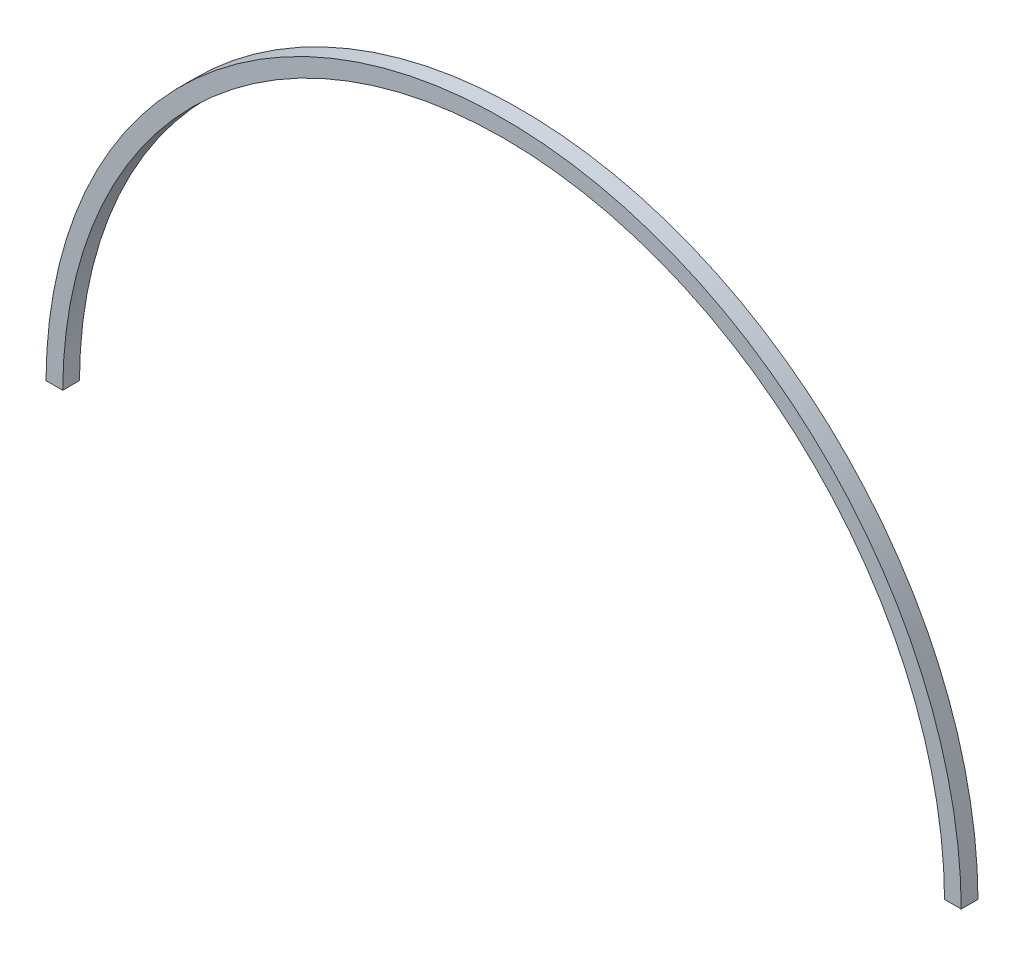
from build123d import *

# Parameters (mm, degrees)
EXTRUDE_1_DEPTH = 4


with BuildPart() as part:
    # 草图1 → 凸台-拉伸1 (new, symmetric)
    with BuildSketch(Plane.XY):
        with BuildLine():
            Line((1.002283117, 1), (9.002369682, 1))
            ThreePointArc((9.002369682, 1), (220, 211), (430.997630318, 1))
            Line((430.997630318, 1), (438.997716883, 1))
            ThreePointArc((438.997716883, 1), (220, 219), (1.002283117, 1))
        make_face()
    extrude(amount=EXTRUDE_1_DEPTH, both=True)


solid = part.part
